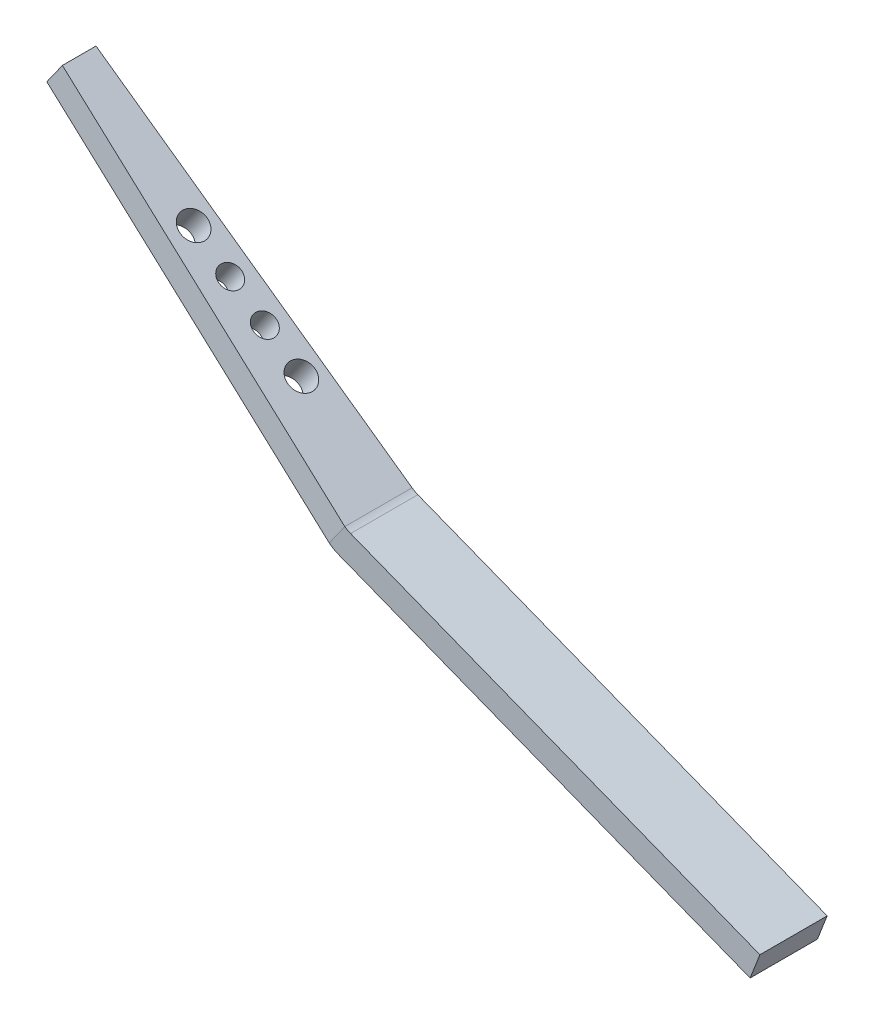
SolidWorks part; units mm, degrees
ref_plane "前视基准面" through (0, 0, 0) normal (0, 0, 1) x (1, 0, 0)
ref_plane "上视基准面" through (0, 0, 0) normal (0, 1, 0) x (1, 0, 0)
ref_plane "右视基准面" through (0, 0, 0) normal (1, 0, 0) x (0, 0, -1)
sketch "草图1" plane through (0, 0, 0) normal (0, 0, 1) x (1, 0, 0)
  line L0 (-156.5525, 182.2852) -> (-144.9682, 198.5887) construction
  line L1 (13.8693, 98.0078) -> (19.1595, 111.5352) construction
  line L2 (-70.4205, 151.9363) -> (16.324, 118.0128) construction
  line L3 (-137.9962, 199.7685) -> (-71.4955, 152.517) construction
  line L4 (-145.5474, 197.7735) -> (-142.0721, 202.6646)
  line L5 (18.7953, 110.6039) -> (20.9806, 116.1918)
  line L6 (-70.3058, 151.8914) -> (20.9806, 116.1918)
  line L7 (-142.0721, 202.6646) -> (-71.5958, 152.5883)
  line L8 (-145.5474, 197.7735) -> (-74.469, 147.2694)
  line L9 (-73.179, 146.5726) -> (18.7953, 110.6039)
  line L12 (-141.4715, 194.8775) -> (-74.9708, 147.6259) construction
  line L13 (-137.9962, 199.7685) -> (-71.4955, 152.517) construction
  line L14 (-70.4205, 151.9363) -> (16.324, 118.0128) construction
  line L15 (-72.6058, 146.3484) -> (14.1387, 112.425) construction
  arc A0 (-73.179, 146.5726) -> (-74.469, 147.2694) centre (-70.9937, 152.1605) cw
  arc A1 (-70.3058, 151.8914) -> (-71.5958, 152.5883) centre (-68.1206, 157.4793) cw
  dimension "D1" = 6
  dimension "D2" = 6
ref_plane "基准面4" through (-137.9962, 199.7685, 0) normal (0.8152, -0.5792, 0) x (0, 0, -1)
extrude "凸台-拉伸1" add sketch "草图1" along normal blind 15
sketch "草图3" plane through (48.0266, 67.5916, 0) normal (0.5792, 0.8152, 0) x (0.8152, -0.5792, 0)
  line L0 (-233.2, -7.5) -> (-146.7446, -15)
  line L3 (-233.2, -15) -> (-233.2, 0) construction
  line L4 (-146.7446, -15) -> (-233.2, -15)
  line L5 (-233.2, -15) -> (-233.2, -7.5)
extrude "切除-拉伸1" cut sketch "草图3" against normal blind 20
hole_wizard "大小mm 暗销孔1" positions "草图4" profile "草图5" hole size "Ø6.0" standard "GB" end condition through all
sketch "草图4" plane through (48.0266, 67.5916, 0) normal (0.5792, 0.8152, 0) x (0.8152, -0.5792, 0)
  point P0 (-200.5235, -4.8708)
  point P3 (-171.0401, -4.8708)
sketch "草图5" plane through (-115.435, 183.7379, 4.8708) normal (0, 0, 1) x (-0.8152, 0.5792, 0)
  line L0 (0, 0) -> (0, 77.0585)
  line L1 (0, 77.0585) -> (3, 77.0585)
  line L2 (3, 77.0585) -> (3, 0)
  line L5 (3, 0) -> (0, 0)
  line L11 (0, -6.35) -> (0, 107.95) construction
  dimension "通孔孔直径" = 6
  dimension "通孔孔深度" = 77.0585
hole_wizard "M6 螺纹孔1" positions "草图6" profile "草图7" tap size "M6" standard "GB" end condition through all
sketch "草图6" plane through (48.0266, 67.5916, 0) normal (0.5792, 0.8152, 0) x (0.8152, -0.5792, 0)
  point P0 (-190.5235, -4.8708)
  point P3 (-181.0401, -4.8708)
sketch "草图7" plane through (-107.2833, 177.9457, 4.8708) normal (0, 0, 1) x (-0.8152, 0.5792, 0)
  line L0 (0, 0) -> (0, 77.0585)
  line L1 (0, 77.0585) -> (2.5, 77.0585)
  line L2 (2.5, 77.0585) -> (2.5, 0)
  line L5 (2.5, 0) -> (0, 0)
  line L11 (0, -6.35) -> (0, 107.95) construction
  dimension "通孔螺纹孔钻头直径" = 5
  dimension "通孔螺纹孔钻头深度" = 77.0585
cosmetic thread "孔螺蚊线1" parameters "D2"=6
cosmetic thread "孔螺蚊线2" parameters "D2"=6
